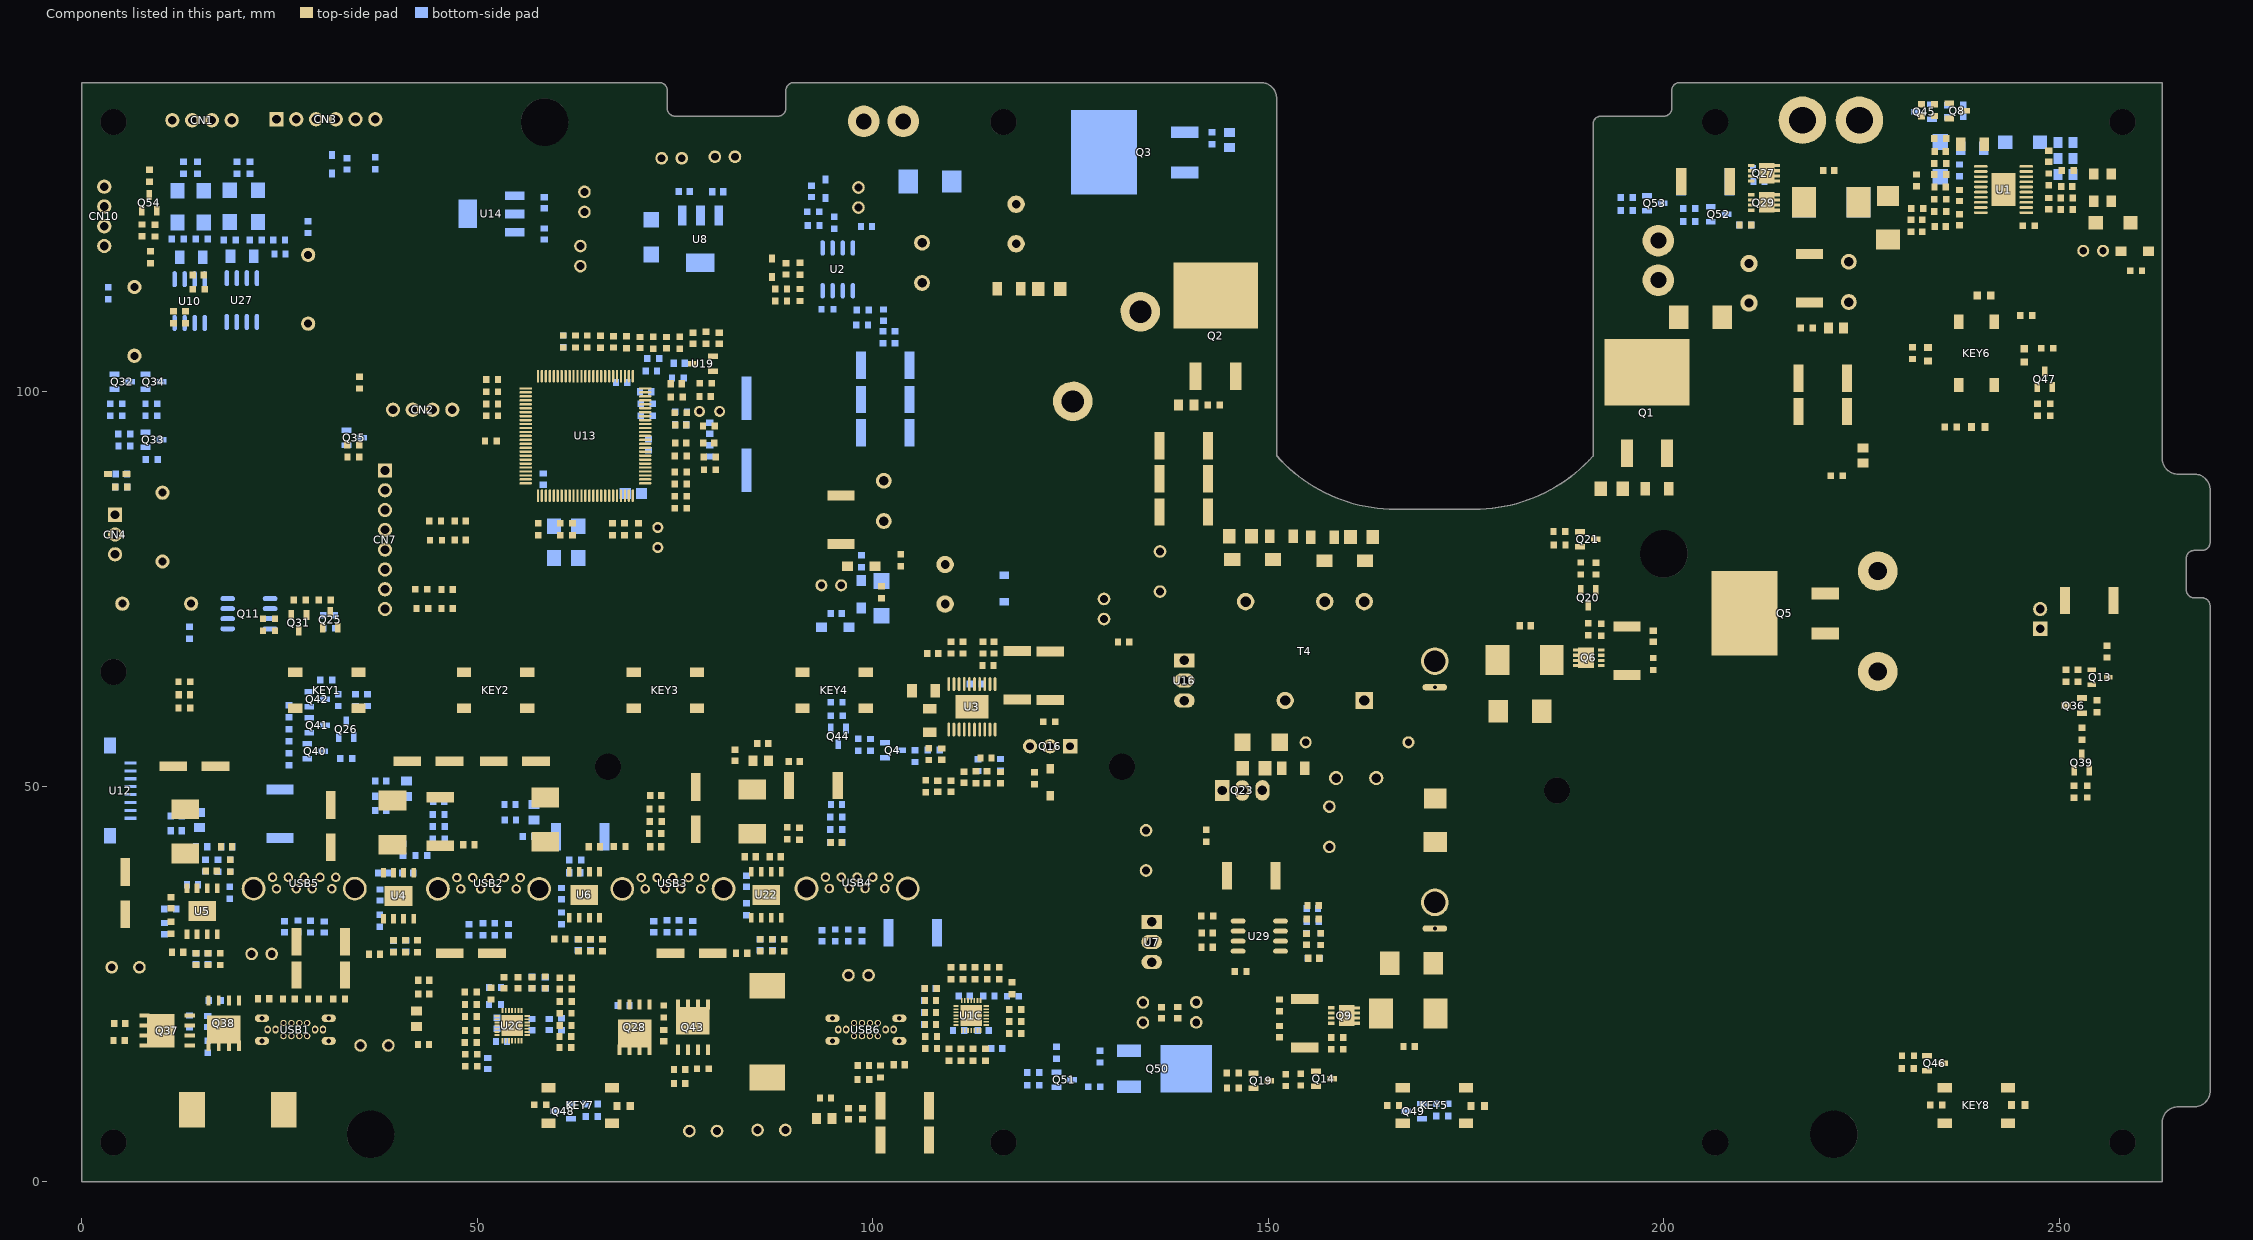
[diagram p0: the components of this part, seen from the top]
# Altium PCB MISC84402.PcbDoc (part 10 of 12)
Units mm, origin at the board's own origin, x right, y up, seen from the top; angles counter-clockwise.
Board outline 269.06 x 139 mm, 4 copper layers (TOP, GND02, PWR03, BOTTOM), stack 0.732 mm thick; 694 components, 428 nets, 1859 pads, 1384 vias.

## Polygon pours and split planes (outlines as drawn) (continued)
NETQ5_3 on TOP "BottomLayer-No Net" (solid, remove dead copper, pour order 1012): 27 vertices, not listed, extent 216.332,73.355 223.444,103.784
NETC10_1 on TOP "BottomLayer-No Net" (solid, remove dead copper, pour order 1011): 58 vertices, not listed, extent 199.314,56.464 231.394,94.64
+12V on TOP "BottomLayer-No Net" (solid, remove dead copper, pour order 1010): 18 vertices, not listed, extent 144.983,22.2 146.634,23.368
NetC75_1 on TOP "BottomLayer-No Net" (solid, remove dead copper, pour order 1009): 26 vertices, not listed, extent 161.011,72.466 171.348,80.518
GND on TOP "BottomLayer-No Net" (solid, remove dead copper, pour order 1008): 30 vertices, not listed, extent 194.513,114.935 212.496,121.768
BATB+ on TOP "BottomLayer-No Net" (solid, remove dead copper, pour order 1007): 18 vertices, not listed, extent 193.548,107.544 204.038,115.494
B+ on TOP "BottomLayer-No Net" (solid, remove dead copper, pour order 1006): 26 vertices, not listed, extent 192.329,97.739 215.163,113.487
+VCC_BAT on TOP "BottomLayer-No Net" (solid, remove dead copper, pour order 1005): 18 vertices, not listed, extent 96.952,118.415 98.908,124.104
+VCC_BAT on TOP "BottomLayer-No Net" (solid, remove dead copper, pour order 1004): 18 vertices, not listed, extent 116.053,80.696 118.212,82.931
NetC75_1 on TOP "BottomLayer-No Net" (solid, remove dead copper, pour order 1002): 18 vertices, not listed, extent 132.537,31.826 136.906,40.894
NetD13_2 on TOP "BottomLayer-No Net" (solid, remove dead copper, pour order 1001): 18 vertices, not listed, extent 154.661,72.111 158.725,80.061
+24V on TOP "Bottom Layer-No Net 2" (hatched 90Degree grid 0.203 track 0.254, remove dead copper, pour order 1431): 239.395,122.682 240.665,122.682 240.919,122.428 240.919,121.539 240.792,121.412 240.411,121.031 239.649,121.031 239.522,121.031 239.268,121.285 239.268,122.555 239.395,122.682
GND on TOP "TOP-No Net 1" (solid, remove dead copper, pour order 1490): 225.044,103.886 225.552,103.378 225.552,95.758 224.155,94.361 222.25,94.361 221.107,95.504 221.107,103.632 221.361,103.886
NETQ5_3 on TOP "Bottom Layer-No Net 2" (solid, remove dead copper, pour order 1439): 219.456,103.759 218.313,103.759 218.186,103.886 218.186,104.003 217.99,104.198 216.339,104.198 216.154,104.013 216.154,95.377 216.408,95.123 219.456,95.123 219.71,95.377 219.71,103.505 219.456,103.759
NETC33_1 on TOP "TOP-No Net 1" (solid, remove dead copper, pour order 1489): 137.541,133.604 142.869,133.604 143.275,133.198 143.536,132.937 143.536,129.159 143.536,129.013 143.325,128.802 143.275,128.752 142.475,128.752 137.916,128.752 137.668,129 137.668,129.413 137.668,133.477 137.541,133.604
GND on TOP "TOP-No Net 1" (solid, remove dead copper, pour order 1480): 43.688,26.797 45.085,26.797 45.593,26.289 45.72,26.162 45.72,25.019 45.72,16.891 45.466,16.637 45.212,16.383 43.942,16.383 43.561,16.764 43.561,18.263 43.561,26.67 43.688,26.797
VOUT2 on TOP "TOP-No Net 1" (solid, remove dead copper, pour order 1479): 24 vertices, not listed, extent 32.258,21.082 42.672,32.534
NETC115_1 on TOP "TOP-No Net 1" (solid, remove dead copper, pour order 1478): 37 vertices, not listed, extent 22.86,5.715 43.053,20.32
NETC77_1 on TOP "TOP-No Net 1" (solid, remove dead copper, pour order 1476): 25 vertices, not listed, extent 11.1,45.847 20.701,53.213
NetC3_2 on TOP "TOP-No Net 1" (solid, remove dead copper, pour order 1474): 22 vertices, not listed, extent 10.922,36.576 14.986,43.053
GND on TOP "TOP-No Net 1" (solid, remove dead copper, pour order 1465): 26 vertices, not listed, extent 128.143,72.009 138.938,95.377
+12V on TOP "TOP-No Net 1" (solid, remove dead copper, pour order 1463): 17 vertices, not listed, extent 127.635,58.097 141.429,71.922
+24V on TOP "TOP-+24V 3" (solid, remove dead copper, pour order 1558): 84.862,32.731 84.608,32.477 83.708,32.477 83.084,31.852 83.084,28.54 82.957,28.413 82.068,28.413 81.814,28.667 81.814,32.411 83.404,34.001 84.735,34.001 84.862,33.874
NETC199_2 on TOP "TOP-No Net" (solid, remove dead copper, pour order 1529): 26 vertices, not listed, extent 89.078,34.214 96.164,52.095
NETC170_2 on TOP "TOP-No Net" (solid, remove dead copper, pour order 1524): 19 vertices, not listed, extent 66.218,34.646 72.542,44.348
NETC49_2 on TOP "TOP-No Net" (solid, remove dead copper, pour order 1519): 48.412,43.764 43.002,43.764 42.494,43.256 42.494,34.29 42.951,33.833 49.632,33.833 49.962,34.163 49.962,39.218 48.539,40.64 48.539,43.637
NETD62_2 on TOP "Top Layer-No Net 1" (solid, remove dead copper, pour order 1515): 24 vertices, not listed, extent 144.932,72.212 153.06,80.34
GND on TOP "TOP-No Net" (solid, remove dead copper, pour order 1525): 17 vertices, not listed, extent 128.659,67.92 133.434,74.955
+VCC_BAT on TOP "TOP-No Net" (solid, remove dead copper, pour order 1516): 24 vertices, not listed, extent 134.45,65.075 147.303,80.34
GND on TOP "TOP-GND" (solid, pour order 1560): 119 vertices, not listed, extent 73.051,3.521 86.005,18.253
NETC107_1 on TOP "TOP-NETC107_1" (solid, pour order 1520): 86.894,3.775 86.894,7.839 84.354,10.379 84.354,15.332 84.735,15.713 93.371,15.713 93.625,15.459 93.625,4.664 92.355,3.394 87.275,3.394 86.894,3.775
NETC86_2 on TOP "TOP-NETC86_2" (solid, pour order 1526): 20 vertices, not listed, extent 11.202,5.68 20.028,21.047
NETC82_2 on TOP "TOP-NETC82_2" (solid, pour order 1530): 48 vertices, not listed, extent 68.987,18.634 89.942,27.397
NetC17_2 on TOP "TOP-NETC151_1" (solid, pour order 1537): 83.338,42.002 82.957,42.383 82.957,45.177 83.084,45.304 86.386,45.304 86.513,45.177 86.513,42.51 86.132,42.129 86.132,40.478 86.005,40.351 84.862,40.351 84.735,40.478 84.735,41.748 84.481,42.002 83.338,42.002
NETC95_1 on TOP "TOP-NETC95_1" (solid, remove dead copper, pour order 1540): 33 vertices, not listed, extent 56.287,46.447 61.367,54.194
NetC8_2 on TOP "TOP-NETC66_1" (solid, pour order 1541): 62.002,40.097 58.319,40.097 56.795,41.621 56.795,44.161 57.176,44.542 60.859,44.542 63.399,42.002 63.399,37.938 63.272,37.811 62.383,37.811 62.256,37.938 62.256,39.843 62.002,40.097
NetC7_2 on TOP "TOP-NETC58_1" (solid, pour order 1542): 18 vertices, not listed, extent 37.364,38.446 41.301,44.034
+13.6V on TOP "TOP-+13.6V" (solid, pour order 1543): 166.904,24.603 164.11,24.603 163.983,24.73 163.983,29.175 164.11,29.302 166.904,29.302 167.031,29.175 167.031,24.73 166.904,24.603
+13.6V on TOP "TOP-+13.6V 2" (solid, pour order 1544): 183.414,62.576 186.208,62.576 186.335,62.449 186.335,57.75 186.208,57.623 183.414,57.623 183.287,57.75 183.287,62.449 183.414,62.576
NETQ9_1 on TOP "TOP-NETQ9_1" (solid, pour order 1545): 150.775,22.825 150.775,25.873 150.902,26 158.268,26 158.395,25.873 158.395,20.666 158.268,20.539 156.49,20.539 156.363,20.666 156.363,22.19 156.236,22.317 152.807,22.317 152.426,22.698 150.902,22.698 150.775,22.825
NETQ6_1 on TOP "TOP-NETQ6_1" (solid, pour order 1546): 199.162,62.703 191.923,62.703 191.669,62.957 191.669,66.64 191.796,66.767 197.511,66.767 197.638,66.64 197.638,65.243 197.765,65.116 199.162,65.116 199.289,64.989 199.289,62.83 199.162,62.703
NETC48_2 on TOP "TOP-NETC48_2" (solid, pour order 1548): 122 vertices, not listed, extent 167.92,57.75 180.874,71.085
NETC48_1 on TOP "TOP-NETC48_1" (solid, pour order 1549): 51 vertices, not listed, extent 167.92,54.448 191.161,69.561
NETC47_2 on TOP "TOP-NETC47_2" (solid, pour order 1550): 147 vertices, not listed, extent 168.047,16.221 181.001,38.827
NETC47_1 on TOP "TOP-NETC47_1" (solid, pour order 1551): 22 vertices, not listed, extent 158.903,16.221 172.873,32.858
B+ on TOP "TOP-B+" (solid, pour order 1553): 175.794,44.161 175.794,40.732 175.667,40.605 168.301,40.605 168.174,40.732 168.174,44.161 168.301,44.288 175.667,44.288 175.794,44.161
+24V on TOP "TOP-+24V 1" (solid, remove dead copper, pour order 1556): 57 vertices, not listed, extent 5.106,17.11 13.615,31.969
+24V on TOP "TOP-+24V 2" (solid, remove dead copper, pour order 1557): 35.459,27.524 35.078,27.905 35.078,32.223 36.729,33.874 38.253,33.874 38.38,33.747 38.38,32.477 38.126,32.223 37.491,32.223 36.798,31.53 36.774,31.53 36.774,31.506 36.602,31.334 36.602,27.524 35.459,27.524
+24V on TOP "TOP-+24V 4" (solid, remove dead copper, pour order 1559): 59.345,28.413 58.933,28.825 58.933,33.852 59.081,34.001 61.748,34.001 61.875,33.874 61.875,32.731 61.621,32.477 60.351,32.477 60.097,32.223 60.097,28.54 59.97,28.413 59.345,28.413
GND on TOP "TOP-GND 1" (solid, pour order 1561): 121 vertices, not listed, extent 1.55,17.11 4.471,28.413
GND on TOP "TOP-GND 3" (solid, pour order 1562): 20.219,24.349 20.219,21.555 20.092,21.428 17.044,21.428 16.917,21.555 16.917,24.222 17.171,24.476 20.092,24.476 20.219,24.349
GND on TOP "TOP-GND 4" (solid, pour order 1563): 145.441,45.177 145.568,45.05 145.568,36.541 145.441,36.414 143.409,36.414 143.155,36.668 143.155,45.05 143.282,45.177 145.441,45.177
GND on TOP "TOP-GND 5" (solid, pour order 1564): 150.933,15.332 150.648,15.617 150.648,18.634 150.775,18.761 152.172,18.761 152.299,18.634 152.299,17.745 152.426,17.618 156.49,17.618 156.617,17.491 156.617,15.459 156.49,15.332 150.933,15.332
GND on TOP "TOP-GND 7" (solid, pour order 1565): 199.543,69.307 199.416,69.18 193.193,69.18 193.066,69.307 193.066,70.069 192.939,70.196 191.542,70.196 191.415,70.323 191.415,71.974 191.542,72.101 199.289,72.101 199.543,71.847 199.543,69.307
AGND on TOP "TOP-No Net" (solid, remove dead copper, pour order 1521): 48.489,54.966 48.717,54.737 48.717,51.511 48.463,51.257 44.298,51.257 44.044,51.511 44.044,54.839 44.171,54.966
AGND on TOP "TOP-No Net" (solid, remove dead copper, pour order 1531): 54.074,54.966 54.302,54.737 54.302,51.511 54.048,51.257 49.883,51.257 49.629,51.511 49.629,54.839 49.756,54.966
AGND on TOP "TOP-No Net" (solid, remove dead copper, pour order 1534): 77.318,47.041 80.965,47.041 81.335,46.671 81.335,42.524 81.102,42.291 76.77,42.291 76.429,42.633 76.429,46.736 76.683,46.99 76.733,47.041 77.318,47.041
NETC41_2 on TOP "TOP-No Net 1" (solid, pour order 1464): 229.997,137.414 230.632,136.779 230.632,122.428 230.124,121.92 222.858,121.92 221.615,123.163 221.615,137.16 221.869,137.414
GND on TOP "TOP-No Net 1" (solid, pour order 1466): 241.808,128.802 244.197,128.802 244.475,128.524 244.475,128.27 244.475,121.666 244.221,121.412 242.189,121.412 241.681,121.412 241.427,121.666 241.427,127.889 241.427,128.675 241.554,128.802 241.808,128.802
NETC41_1 on TOP "TOP-No Net 1" (solid, remove dead copper, pour order 1468): 21 vertices, not listed, extent 211.963,121.793 220.472,137.414
NETQ27_1 on TOP "TOP-No Net 1" (solid, remove dead copper, pour order 1470): 210.947,123.088 210.947,124.993 209.804,124.993 209.296,125.501 209.296,126.39 210.058,127.152 211.328,127.152 211.455,127.279 211.455,128.549 210.947,129.057 208.063,129.057 206.457,127.451 206.457,123.388 206.756,123.088
B+ on TOP "TOP-No Net 1" (solid, pour order 1471): 125.222,135.763 136.271,135.763 136.525,135.509 136.779,135.255 136.779,134.493 136.779,125.349 136.271,124.841 136.017,124.587 132.08,124.587 125.349,124.587 124.968,124.968 124.968,135.255 124.968,135.509 125.222,135.763
B+ on TOP "TOP-No Net 1" (solid, remove dead copper, pour order 1472): 30 vertices, not listed, extent 108.331,122.174 132.588,135.763
GND on TOP "TOP-No Net 1" (solid, remove dead copper, pour order 1475): 18 vertices, not listed, extent 116.586,115.189 124.714,121.539
VBUSC-1 on TOP "TOP-No Net 1" (solid, remove dead copper, pour order 1482): 27 vertices, not listed, extent 96.139,3.429 108.712,18.923
VOUT1 on TOP "TOP-No Net 1" (solid, remove dead copper, pour order 1483): 21 vertices, not listed, extent 94.234,3.342 102.362,11.684
GND on TOP "TOP-No Net 1" (solid, remove dead copper, pour order 1484): 23 vertices, not listed, extent 94.107,8.95 99.06,14.859
BATA+ on TOP "Bottom Layer-No Net 2" (solid, remove dead copper, pour order 1434): 102.997,138.43 110.363,138.43 110.744,138.049 110.744,131.064 110.49,130.81 102.743,130.81 102.235,131.318 102.235,138.176 102.489,138.43 102.997,138.43
GND on TOP "Bottom Layer-No Net 2" (solid, remove dead copper, pour order 1437): 28 vertices, not listed, extent 92.583,116.713 110.617,138.811
+24V on TOP "TOP-+24V" (solid, remove dead copper, pour order 1555): 21 vertices, not listed, extent 67.183,3.648 77.877,20.574
NETCON1_2 on TOP "BottomLayer-No Net" (solid, remove dead copper, pour order 1000): 19 vertices, not listed, extent 245.643,71.526 251.612,75.641
NetR124_2 on TOP "BottomLayer-No Net" (solid, remove dead copper, pour order 1001): 18 vertices, not listed, extent 255.219,67.412 258.115,75.667
+24V on TOP "BottomLayer-No Net" (solid, remove dead copper, pour order 1002): 25 vertices, not listed, extent 3.785,29.667 9.957,35.662
+24V on TOP "BottomLayer-No Net" (solid, remove dead copper, pour order 1003): 31 vertices, not listed, extent 77.876,28.067 84.938,34.011
+24V on TOP "BottomLayer-No Net" (solid, remove dead copper, pour order 1005): 47 vertices, not listed, extent 30.099,27.457 38.481,44.221
NETC10_1 on TOP "BottomLayer-No Net" (solid, remove dead copper, pour order 1000): 22 vertices, not listed, extent 199.365,85.852 213.131,94.64
GND on GND02 "BottomLayer-No Net" (solid, remove dead copper, pour order 1004): 196 vertices, not listed, extent 0.33,0.305 273.406,158.775
AGND on GND02 "BottomLayer-No Net" (solid, remove dead copper, pour order 1003): 55 vertices, not listed, extent 8.712,24.155 104.267,55.524
B+ on GND02 "TOP-No Net 1" (solid, remove dead copper, pour order 1498): 123.063,122.809 125.349,125.095 133.096,125.095 133.858,125.857 133.858,135.128 132.995,135.991 109.956,135.991 109.601,135.636 109.601,129.826 107.823,128.048 107.823,124.841 109.855,122.808
NETC33_1 on GND02 "TOP-No Net 1" (solid, remove dead copper, pour order 1497): 25 vertices, not listed, extent 125.603,102.362 144.145,136.271
GND on GND02 "Bottom Layer-No Net 2" (solid, remove dead copper, pour order 1438): 144 vertices, not listed, extent -0.889,15.799 123.266,140.233
+13.6V on GND02 "BottomLayer-No Net" (solid, remove dead copper, pour order 1004): 50 vertices, not listed, extent 226.187,56.718 257.708,120.955
GND on GND02 "BottomLayer-No Net" (solid, remove dead copper, pour order 1000): 27 vertices, not listed, extent 65.557,21.946 111.836,28.575
"VDD 3.3V" on PWR03 "BottomLayer-No Net" (solid, remove dead copper, pour order 1015): 30 vertices, not listed, extent 42.316,67.285 91.44,83.998
"VDD 3.3V" on PWR03 "BottomLayer-No Net" (solid, remove dead copper, pour order 1014): 22 vertices, not listed, extent 0.33,61.011 51.054,112.852
+13.6V on PWR03 "BottomLayer-No Net" (solid, remove dead copper, pour order 1013): 31 vertices, not listed, extent 93.269,44.983 143.713,105.207
AGND on PWR03 "BottomLayer-No Net" (solid, remove dead copper, pour order 1012): 68 vertices, not listed, extent 0.533,26.314 108.331,64.948
+24V on PWR03 "BottomLayer-No Net" (solid, remove dead copper, pour order 1011): 90 vertices, not listed, extent -0.889,-6.426 272.263,113.055
VDD1 on PWR03 "BottomLayer-No Net" (solid, remove dead copper, pour order 1010): 26 vertices, not listed, extent 52.095,80.061 72.923,105.385
"VDD 3.3V" on PWR03 "BottomLayer-No Net" (solid, remove dead copper, pour order 1009): 70 vertices, not listed, extent 0.33,77.749 98.831,144.018
NetC75_1 on PWR03 "BottomLayer-No Net" (solid, remove dead copper, pour order 1018): 42 vertices, not listed, extent 133.655,31.725 174.828,74.016
B+ on PWR03 "BottomLayer-No Net" (solid, remove dead copper, pour order 1017): 69 vertices, not listed, extent 109.372,37.922 220.929,141.58
BAT1+ on PWR03 "Bottom Layer-No Net 2" (solid, remove dead copper, pour order 1447): 147.005,62.128 163.418,62.128 167.924,57.887 168.427,57.413 168.427,53.716 168.427,43.006 166.841,41.513 165.105,39.878 155.79,39.878 146.804,39.878 145.872,40.755 145.872,61.323 145.973,61.418 146.728,62.128 147.005,62.128
GND on PWR03 "Bottom Layer-No Net 2" (solid, remove dead copper, pour order 1451): 263.627,114.884 205.334,114.884 204.419,115.799 203.2,117.018 196.723,117.018 191.033,117.018 190.195,117.856 190.195,135.915 195.656,141.376 262.661,141.376 264.211,139.827 264.211,115.468 263.627,114.884
BATA+ on PWR03 "Bottom Layer-No Net 2" (solid, remove dead copper, pour order 1458): 103.251,138.43 110.236,138.43 110.49,138.176 110.49,131.191 110.109,130.81 102.362,130.81 102.108,131.064 102.108,138.176 102.362,138.43 103.251,138.43
GND on PWR03 "Bottom Layer-No Net 2" (solid, remove dead copper, pour order 1459): 17 vertices, not listed, extent 90.424,117.348 108.204,139.446
+24V on BOTTOM "BottomLayer-No Net" (solid, remove dead copper, pour order 1005): 18 vertices, not listed, extent 54.026,28.245 60.223,30.378
B+ on BOTTOM "BottomLayer-No Net" (solid, remove dead copper, pour order 1024): 23 vertices, not listed, extent 195.021,104.496 214.401,112.497
+24V on BOTTOM "BottomLayer-No Net" (solid, remove dead copper, pour order 1023): 28 vertices, not listed, extent 220.802,77.292 238.76,113.335
NETC10_1 on BOTTOM "BottomLayer-No Net" (solid, remove dead copper, pour order 1022): 26 vertices, not listed, extent 195.478,73.304 215.316,94.945
+12V on BOTTOM "BottomLayer-No Net" (solid, remove dead copper, pour order 1021): 30 vertices, not listed, extent 175.819,2.134 243.281,26.086
+VCC_BAT on BOTTOM "BottomLayer-No Net" (solid, remove dead copper, pour order 1020): 29 vertices, not listed, extent 115.291,73 137.947,83.617
+12V on BOTTOM "BottomLayer-No Net" (solid, remove dead copper, pour order 1019): 84 vertices, not listed, extent 119.964,2.134 262.28,117.881
+13.6V on BOTTOM "BottomLayer-No Net" (solid, remove dead copper, pour order 1018): 78 vertices, not listed, extent 115.722,24.003 247.396,62.738
+13.6V-F on BOTTOM "BottomLayer-No Net" (solid, remove dead copper, pour order 1017): 22 vertices, not listed, extent 103.734,91.542 127.787,115.062
GND on BOTTOM "BottomLayer-No Net" (solid, remove dead copper, pour order 1001): 36 vertices, not listed, extent 72.822,86.563 86.868,102.362
VCC9V on BOTTOM "BottomLayer-No Net" (solid, remove dead copper, pour order 1018): 67 vertices, not listed, extent 36.017,120.802 81.559,137.846
GND on BOTTOM "BottomLayer-No Net" (solid, remove dead copper, pour order 1017): 30 vertices, not listed, extent 71.12,120.777 76.556,130.353
GND on BOTTOM "BottomLayer-No Net" (solid, remove dead copper, pour order 1016): 22 vertices, not listed, extent 80.67,124.46 84.48,130.581
NetC85_2 on BOTTOM "BottomLayer-No Net" (solid, remove dead copper, pour order 1015): 41 vertices, not listed, extent 70.333,114.884 80.721,130.327
"VDD 3.3V" on BOTTOM "BottomLayer-No Net" (solid, remove dead copper, pour order 1014): 30 vertices, not listed, extent 47.498,120.396 73.355,124.739
NETCN4_3 on BOTTOM "BottomLayer-No Net" (solid, remove dead copper, pour order 1013): 17 vertices, not listed, extent 2.692,71.73 11.76,80.518
NETC77_1 on BOTTOM "BottomLayer-No Net" (solid, remove dead copper, pour order 1012): 21 vertices, not listed, extent 12.192,45.745 19.837,50.698
NetC101_2 on BOTTOM "BottomLayer-No Net" (solid, remove dead copper, pour order 1011): 47 vertices, not listed, extent 12.192,40.31 27.127,50.521
NetC105_2 on BOTTOM "BottomLayer-No Net" (solid, remove dead copper, pour order 1010): 20 vertices, not listed, extent 37.465,50.14 41.986,54
NETC57_2 on BOTTOM "BottomLayer-No Net" (solid, remove dead copper, pour order 1009): 34 vertices, not listed, extent 38.024,42.291 46.787,50.927
NETC95_1 on BOTTOM "BottomLayer-No Net" (solid, remove dead copper, pour order 1008): 26 vertices, not listed, extent 54.407,47.244 60.503,52.07
NetC117_2 on BOTTOM "BottomLayer-No Net" (solid, remove dead copper, pour order 1007): 34 vertices, not listed, extent 54.432,40.361 62.078,46.457
+13.6V on BOTTOM "BottomLayer-No Net" (solid, remove dead copper, pour order 1003): 23 vertices, not listed, extent 97.815,86.995 104.673,105.385
GND on BOTTOM "BottomLayer-No Net" (solid, remove dead copper, pour order 1027): 19 vertices, not listed, extent 95.504,81.153 102.641,84.912
+5V on BOTTOM "TOP-No Net" (solid, remove dead copper, pour order 1523): 68.682,120.193 68.707,115.443 67.564,114.3 54.737,114.3 53.467,115.57 53.467,120.396 53.721,120.65 56.312,120.65 57.582,119.38 59.853,119.38 60.897,120.424 68.451,120.424
NETQ5_3 on BOTTOM "BottomLayer-No Net" (solid, remove dead copper, pour order 1026): 22 vertices, not listed, extent 205.435,95.199 219.786,103.226
VDD1 on BOTTOM "BottomLayer-No Net" (solid, remove dead copper, pour order 1023): 22 vertices, not listed, extent 55.753,103.911 61.366,105.918
"VDD 3.3V" on BOTTOM "BottomLayer-No Net" (solid, remove dead copper, pour order 1022): 18 vertices, not listed, extent 60.096,106.604 61.722,108.737
+5V on BOTTOM "BottomLayer-No Net" (solid, remove dead copper, pour order 1021): 34 vertices, not listed, extent 127.711,15.646 142.138,28.753
GND on BOTTOM "TOP-No Net 1" (solid, remove dead copper, pour order 1508): 204.724,118.11 204.47,117.856 204.47,114.427 204.978,113.919 226.568,113.919 227.584,114.935 227.584,117.602 227.076,118.11
GND on BOTTOM "TOP-No Net 1" (solid, remove dead copper, pour order 1510): 22 vertices, not listed, extent 133.477,77.724 138.938,95.377
GND on BOTTOM "TOP-No Net 1" (solid, remove dead copper, pour order 1509): 23 vertices, not listed, extent 99.441,115.697 124.714,125.095
NETC40_2 on BOTTOM "TOP-No Net 1" (solid, remove dead copper, pour order 1501): 20 vertices, not listed, extent 107.696,70.866 118.999,79.375
NETC170_2 on BOTTOM "TOP-No Net" (solid, remove dead copper, pour order 1539): 66.091,46.38 71.145,46.38 71.628,45.898 72.111,45.415 72.111,35.738 72.111,34.976 71.272,34.138 66.269,34.138 65.532,34.874 65.507,34.9 65.507,43.79 65.507,45.796 66.091,46.38
NETC192_2 on BOTTOM "TOP-No Net" (solid, remove dead copper, pour order 1538): 18 vertices, not listed, extent 19.685,33.985 27.559,44.552
NETC49_2 on BOTTOM "BOTTOM-NETC49_2" (solid, pour order 1567): 43.079,41.748 43.206,41.875 44.984,41.875 45.365,42.256 45.365,43.78 45.492,43.907 47.651,43.907 47.778,43.78 47.778,40.986 47.524,40.732 43.206,40.732 43.079,40.859 43.079,41.748
NETD5_2 on BOTTOM "BOTTOM-NETD5_2" (solid, pour order 1569): 134 vertices, not listed, extent 11.456,69.942 14.758,74.387
NETCN4_2 on BOTTOM "BOTTOM-NETCN4_2" (solid, pour order 1572): 19.33,73.752 19.33,69.18 18.949,68.799 15.901,68.799 15.393,69.307 15.393,74.006 15.647,74.26 18.822,74.26 19.33,73.752
NETC48_1 on BOTTOM "BOTTOM-NETC48_1" (solid, pour order 1573): 190.907,69.561 191.161,69.307 191.161,63.338 191.034,63.211 182.144,63.211 178.842,59.909 169.444,59.909 169.19,60.163 169.19,62.957 169.317,63.084 175.286,63.084 181.763,69.561 190.907,69.561
NETC47_1 on BOTTOM "BOTTOM-NETC47_1" (solid, pour order 1574): 163.602,30.064 163.475,29.937 163.475,20.031 163.348,19.904 159.03,19.904 158.903,20.031 158.903,32.731 159.03,32.858 172.746,32.858 172.873,32.731 172.873,30.191 172.746,30.064 163.602,30.064
+12V on BOTTOM "BOTTOM-+12V" (solid, pour order 1576): 42.444,92.04 42.698,92.294 45.619,92.294 45.746,92.167 45.746,90.135 45.111,89.5 42.825,89.5 42.444,89.881 42.444,92.04
AGND on BOTTOM "BOTTOM-AGND" (solid, pour order 1579): 99.899,33.848 102.439,33.848 102.693,33.594 102.693,29.784 102.312,29.403 100.026,29.403 99.772,29.657 99.772,33.721 99.899,33.848
+13.6V-F on BOTTOM "BOTTOM-+24V" (solid, pour order 1581): 14.25,68.799 14.25,67.275 14.123,67.148 12.472,67.148 12.218,67.402 12.218,68.799 12.472,69.053 13.996,69.053 14.25,68.799
GND on BOTTOM "BOTTOM-GND 1" (solid, pour order 1583): 130 vertices, not listed, extent 2.947,24.73 13.488,31.715
GND on BOTTOM "BOTTOM-GND 2" (solid, pour order 1584): 15.647,22.19 16.79,22.19 17.171,22.571 17.171,24.349 17.298,24.476 20.092,24.476 20.219,24.349 20.219,21.047 19.838,20.666 15.647,20.666 15.52,20.793 15.52,22.063 15.647,22.19
GND on BOTTOM "BOTTOM-GND 3" (solid, pour order 1585): 107.392,33.848 110.059,33.848 110.44,33.467 110.44,29.657 110.059,29.276 107.392,29.276 107.011,29.657 107.011,33.467 107.392,33.848
GND on BOTTOM "BOTTOM-GND 4" (solid, pour order 1586): 26.061,73.879 26.061,71.339 25.68,70.958 22.124,70.958 21.87,71.212 21.87,74.133 22.124,74.387 25.553,74.387 26.061,73.879
GND on BOTTOM "BOTTOM-GND 6" (solid, pour order 1587): 53.493,124.298 53.493,126.076 53.874,126.457 64.288,126.457 64.669,126.076 64.669,124.425 64.161,123.917 53.874,123.917 53.493,124.298
NETC41_2 on BOTTOM "TOP-No Net 1" (solid, pour order 1485): 229.997,137.414 230.632,136.779 230.632,122.428 230.124,121.92 222.858,121.92 221.615,123.163 221.615,137.16 221.869,137.414